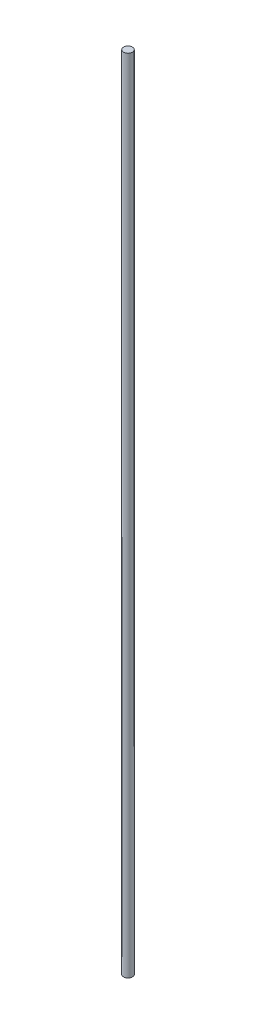
SolidWorks part; units mm, degrees
material "黄铜"
ref_plane "Front Plane" through (0, 0, 0) normal (0, 0, 1) x (1, 0, 0)
ref_plane "Top Plane" through (0, 0, 0) normal (0, 1, 0) x (1, 0, 0)
ref_plane "Right Plane" through (0, 0, 0) normal (1, 0, 0) x (0, 0, -1)
sketch "Sketch1" plane through (0, 0, 0) normal (0, 0, 1) x (1, 0, 0)
  line L0 (0, -6.4416) -> (0, 89.5755) construction
  line L2 (0, 0) -> (-0.5, 0)
  line L3 (0, 0) -> (0, 90)
  line L4 (0, 90) -> (-0.5, 90)
  line L5 (-0.5, 0) -> (-0.5, 90)
  dimension "D1" = 1
  dimension "D2" = 90
revolve "Revolve1" add sketch "Sketch1" angle 360 about L0
